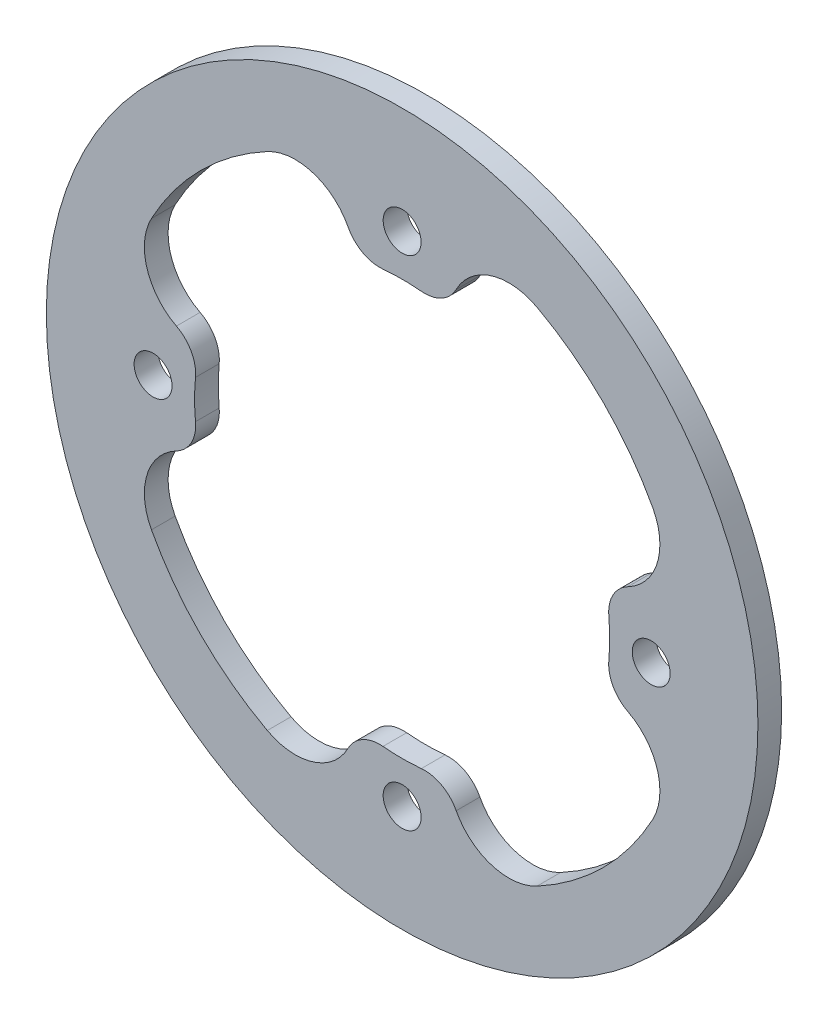
from build123d import *

# Parameters (mm, degrees)
SKETCH_1_R          = 30
EXTRUDE_1_DEPTH     = 2
SKETCH_2_R          = 1.6
CUT_EXTRUDE_1_DEPTH = 10
SKETCH_3_R          = 2.55
CUT_EXTRUDE_2_DEPTH = 10
SKETCH_4_R          = 17.5
CUT_EXTRUDE_3_DEPTH = 10
FILLET_1_R          = 3


with BuildPart() as part:
    # 草图1 → 凸台-拉伸1 (new body)
    with BuildSketch(Plane.XY):
        Circle(SKETCH_1_R)
        with BuildLine():
            Line((4, 16.733200531), (4, 12))
            ThreePointArc((4, 12), (4.527864045, 9.763932023), (6, 8))
            ThreePointArc((6, 8), (7.071067812, 7.071067812), (8, 6))
            ThreePointArc((8, 6), (9.763932023, 4.527864045), (12, 4))
            Line((12, 4), (16.733200531, 4))
            ThreePointArc((16.733200531, 4), (21.025175907, 6.43505412), (21.136674355, 11.368421053))
            ThreePointArc((21.136674355, 11.368421053), (16.970562748, 16.970562748), (11.368421053, 21.136674355))
            ThreePointArc((11.368421053, 21.136674355), (6.43505412, 21.025175907), (4, 16.733200531))
        make_face(mode=Mode.SUBTRACT)
        with BuildLine():
            Line((-4, 16.733200531), (-4, 12))
            ThreePointArc((-4, 12), (-4.527864045, 9.763932023), (-6, 8))
            ThreePointArc((-6, 8), (-7.071067812, 7.071067812), (-8, 6))
            ThreePointArc((-8, 6), (-9.763932023, 4.527864045), (-12, 4))
            Line((-12, 4), (-16.733200531, 4))
            ThreePointArc((-16.733200531, 4), (-21.025175907, 6.43505412), (-21.136674355, 11.368421053))
            ThreePointArc((-21.136674355, 11.368421053), (-16.970562748, 16.970562748), (-11.368421053, 21.136674355))
            ThreePointArc((-11.368421053, 21.136674355), (-6.43505412, 21.025175907), (-4, 16.733200531))
        make_face(mode=Mode.SUBTRACT)
        with BuildLine():
            Line((16.733200531, -4), (12, -4))
            ThreePointArc((12, -4), (9.763932023, -4.527864045), (8, -6))
            ThreePointArc((8, -6), (7.071067812, -7.071067812), (6, -8))
            ThreePointArc((6, -8), (4.527864045, -9.763932023), (4, -12))
            Line((4, -12), (4, -16.733200531))
            ThreePointArc((4, -16.733200531), (6.43505412, -21.025175907), (11.368421053, -21.136674355))
            ThreePointArc((11.368421053, -21.136674355), (16.970562748, -16.970562748), (21.136674355, -11.368421053))
            ThreePointArc((21.136674355, -11.368421053), (21.025175907, -6.43505412), (16.733200531, -4))
        make_face(mode=Mode.SUBTRACT)
        with BuildLine():
            Line((-4, -16.733200531), (-4, -12))
            ThreePointArc((-4, -12), (-4.527864045, -9.763932023), (-6, -8))
            ThreePointArc((-6, -8), (-7.071067812, -7.071067812), (-8, -6))
            ThreePointArc((-8, -6), (-9.763932023, -4.527864045), (-12, -4))
            Line((-12, -4), (-16.733200531, -4))
            ThreePointArc((-16.733200531, -4), (-21.025175907, -6.43505412), (-21.136674355, -11.368421053))
            ThreePointArc((-21.136674355, -11.368421053), (-16.970562748, -16.970562748), (-11.368421053, -21.136674355))
            ThreePointArc((-11.368421053, -21.136674355), (-6.43505412, -21.025175907), (-4, -16.733200531))
        make_face(mode=Mode.SUBTRACT)
    extrude(amount=EXTRUDE_1_DEPTH)

    # 草图2 → 切除-拉伸1 (cut)
    with BuildSketch(Plane.XY.offset(2)):
        with Locations((-21, 0)):
            Circle(SKETCH_2_R)
        with Locations((0, 21)):
            Circle(SKETCH_2_R)
        with Locations((21, 0)):
            Circle(SKETCH_2_R)
        with Locations((0, -21)):
            Circle(SKETCH_2_R)
    extrude(amount=-CUT_EXTRUDE_1_DEPTH, mode=Mode.SUBTRACT)

    # 草图3 → 切除-拉伸2 (cut)
    with BuildSketch(Plane.XY.offset(2)):
        with Locations((0, 6)):
            Circle(SKETCH_3_R)
        with Locations((-6, 0)):
            Circle(SKETCH_3_R)
        with Locations((6, 0)):
            Circle(SKETCH_3_R)
        with Locations((0, -6)):
            Circle(SKETCH_3_R)
    extrude(amount=-CUT_EXTRUDE_2_DEPTH, mode=Mode.SUBTRACT)

    # 草图4 → 切除-拉伸3 (cut)
    with BuildSketch(Plane.XY.offset(2)):
        Circle(SKETCH_4_R)
    extrude(amount=-CUT_EXTRUDE_3_DEPTH, mode=Mode.SUBTRACT)

    # 圆角1
    fillet_1_edges = [part.edges().sort_by_distance(p)[0] for p in [
        (-4.009091698, -17.034587866, 1),
        (4.009091698, 17.034587866, 1),
        (17.034587866, 4.009091698, 1),
        (17.034587866, -4.009091698, 1),
        (4.009091698, -17.034587866, 1),
        (-17.034587866, -4.009091698, 1),
        (-17.034587866, 4.009091698, 1),
        (-4.009091698, 17.034587866, 1),
    ]]
    fillet(fillet_1_edges, radius=FILLET_1_R)


solid = part.part
